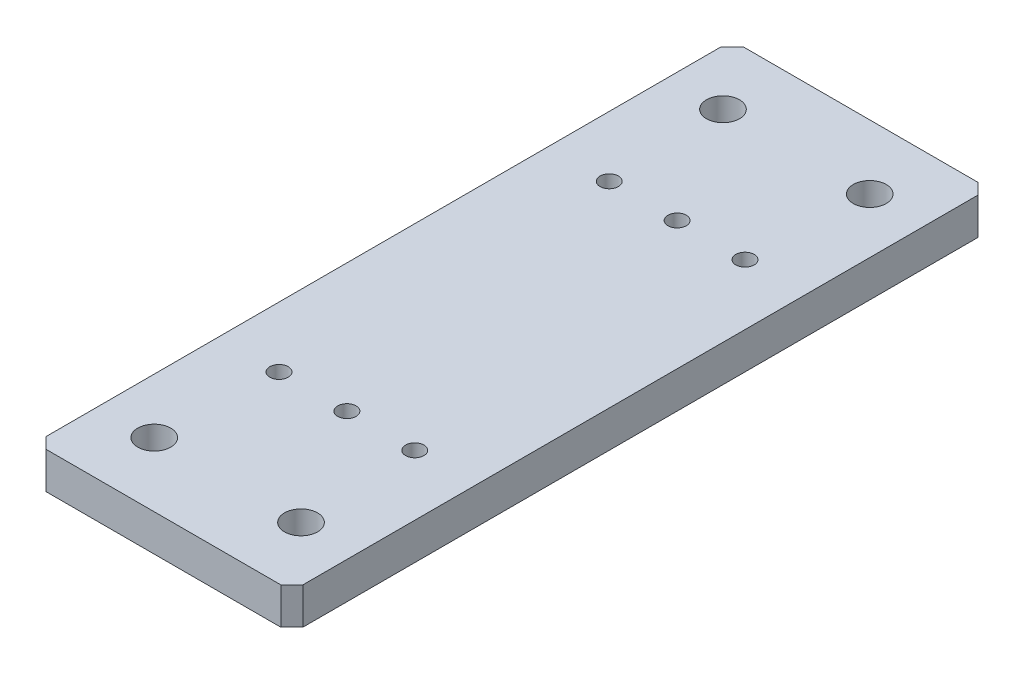
from build123d import *

# Parameters (mm, degrees)
SKETCH_1_W            = 70
SKETCH_1_H            = 190
EXTRUDE_1_DEPTH       = 10
HOLE_WIZARD_M6_1_D    = 5
HOLE_WIZARD_9_0_9_1_D = 9
CHAMFER_1_SIZE        = 3


with BuildPart() as part:
    # 草图1 → 凸台-拉伸1 (new body)
    with BuildSketch(Plane(origin=(0, 0, 0), x_dir=(1, 0, 0), z_dir=(0, 1, 0))):
        Rectangle(SKETCH_1_W, SKETCH_1_H)
    extrude(amount=EXTRUDE_1_DEPTH)

    # M6 螺纹孔1 (through all)
    with Locations(Plane(origin=(0, 10, 0), x_dir=(1, 0, 0), z_dir=(0, 1, 0))):
        with Locations((18.5, 45), (-18.5, 45), (0, 45), (0, -45), (-18.5, -45), (18.5, -45)):
            Hole(HOLE_WIZARD_M6_1_D / 2)

    # Ø9.0 (9) 直径孔1 (through all)
    with Locations(Plane(origin=(0, 10, 0), x_dir=(1, 0, 0), z_dir=(0, 1, 0))):
        with Locations((-20, 77.5), (20, 77.5), (20, -77.5), (-20, -77.5)):
            Hole(HOLE_WIZARD_9_0_9_1_D / 2)

    # 倒角1
    chamfer_1_edges = [part.edges().sort_by_distance(p)[0] for p in [
        (35, 5, 95),
        (-35, 5, 95),
        (-35, 5, -95),
        (35, 5, -95),
    ]]
    chamfer(chamfer_1_edges, length=CHAMFER_1_SIZE)


solid = part.part
